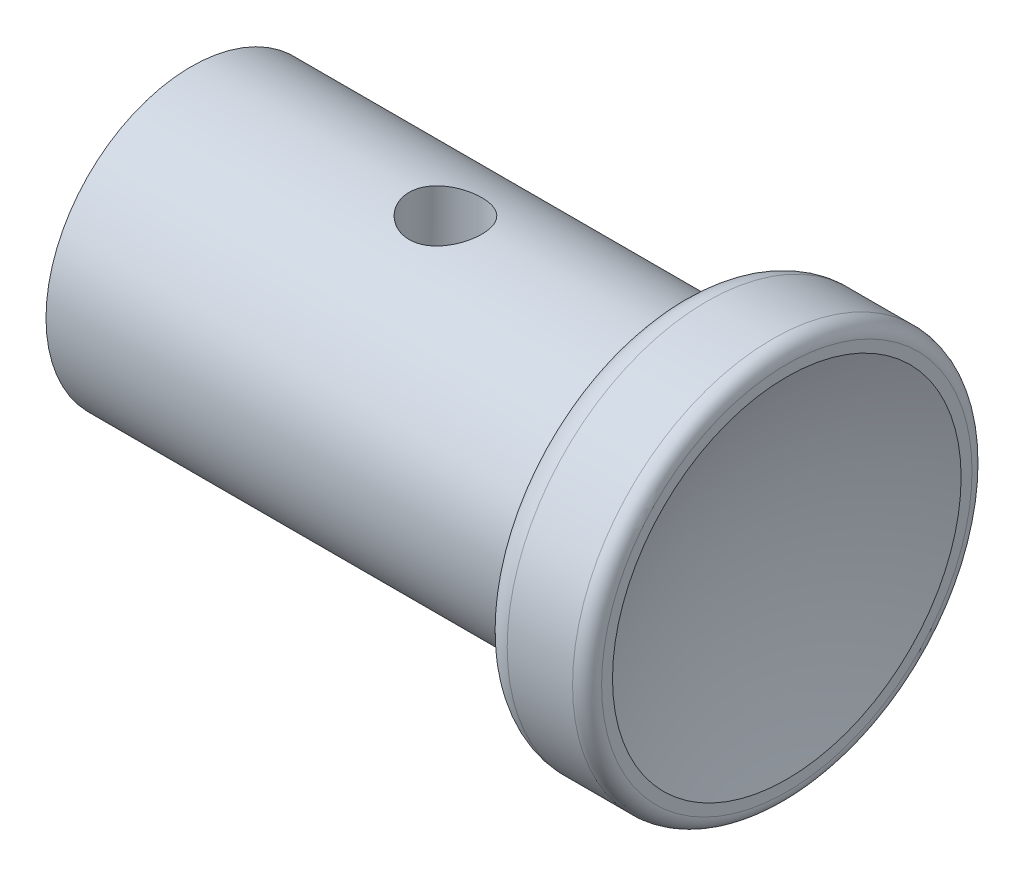
from build123d import *

# Parameters (mm, degrees)
M24_TAPPED_HOLE1_D     = 21
M24_TAPPED_HOLE1_DEPTH = 57
M24_TAPPED_HOLE1_TIP   = 6.3090365
SKETCH4_R              = 5
CUT_EXTRUDE1_DEPTH     = 25
FILLET2_R              = 2
FILLET3_R              = 4


with BuildPart() as part:
    # Sketch1 → Revolve1 (revolve)
    with BuildSketch(Plane.XY, mode=Mode.PRIVATE) as revolve1_sk:
        with BuildLine():
            Line((67, 27.5), (67, 20))
            Line((67, 20), (0, 20))
            Line((0, 20), (0, 0))
            Line((0, 0), (77.589222534, 0))
            ThreePointArc((77.589222534, 0), (78.70107404, 12.20097289), (82, 24))
            Line((82, 24), (82, 27.5))
            Line((82, 27.5), (67, 27.5))
        make_face()
    revolve(revolve1_sk.sketch.rotate(Axis((0, 0, 0), (1, 0, 0)), 90), axis=Axis((0, 0, 0), (1, 0, 0)))

    # M24 Tapped Hole1
    with Locations(Plane.ZY):
        with Locations((0, 0)):
            Hole(M24_TAPPED_HOLE1_D / 2, depth=M24_TAPPED_HOLE1_DEPTH)
            with Locations((0, 0, -(M24_TAPPED_HOLE1_DEPTH + M24_TAPPED_HOLE1_TIP / 2))):  # 118° drill point
                Cone(0, M24_TAPPED_HOLE1_D / 2, M24_TAPPED_HOLE1_TIP, mode=Mode.SUBTRACT)

    # Sketch4 → Cut-Extrude1 (cut, symmetric)
    with BuildSketch(Plane(origin=(0, 0, 0), x_dir=(1, 0, 0), z_dir=(0, 1, 0))):
        with Locations(Location((35, 0, 0), (0, 0, 270))):
            Circle(SKETCH4_R)
    extrude(amount=CUT_EXTRUDE1_DEPTH, both=True, mode=Mode.SUBTRACT)

    # Fillet2
    fillet2_edges = [part.edges().sort_by_distance(p)[0] for p in [
        (82, 0, -27.5),
    ]]
    fillet(fillet2_edges, radius=FILLET2_R)

    # Fillet3
    fillet3_edges = [part.edges().sort_by_distance(p)[0] for p in [
        (67, 0, -27.5),
    ]]
    fillet(fillet3_edges, radius=FILLET3_R)


solid = part.part
